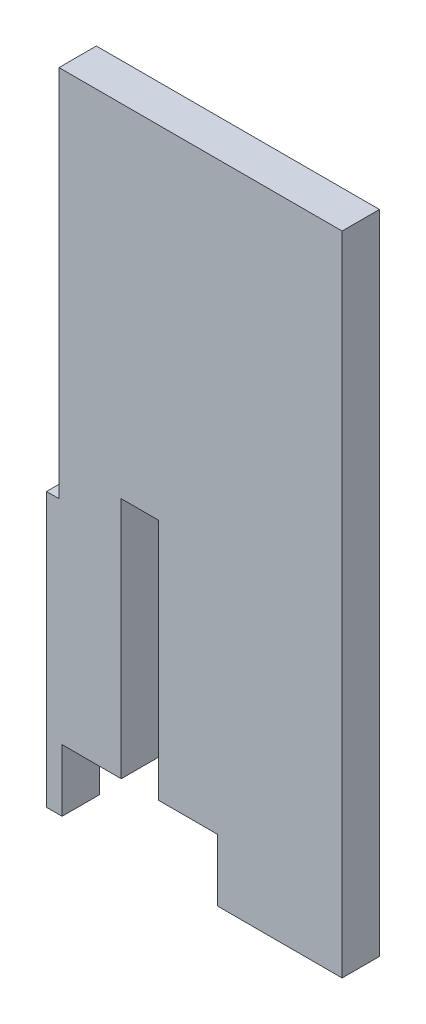
from build123d import *

# Parameters (mm, degrees)
BOSS_EXTRUDE1_DEPTH = 6
SKETCH3_W           = 6
SKETCH3_H           = 60
CUT_EXTRUDE1_DEPTH  = 10
CUT_EXTRUDE2_DEPTH  = 187.01085661


with BuildPart() as part:
    # Sketch1 → Boss-Extrude1 (new body)
    with BuildSketch(Plane.XY):
        Polygon((127.020625139, -33.445286794), (107.020625139, -33.445286794), (107.020625139, 70.514713206), (172.022422952, 70.514713206), (172.022422952, -33.445286794), (152.022422952, -33.445286794), (152.022422952, -23.465104548), (127.020625139, -23.465104548), align=None)
    extrude(amount=BOSS_EXTRUDE1_DEPTH)

    # Sketch3 → Cut-Extrude1 (cut)
    with BuildSketch(Plane(origin=(0, 0, 0), x_dir=(-1, 0, 0), z_dir=(0, 0, -1))):
        with Locations((-139.522422952, -14.485286794)):
            Rectangle(SKETCH3_W, SKETCH3_H)
    extrude(amount=-CUT_EXTRUDE1_DEPTH, mode=Mode.SUBTRACT)

    # Sketch4 → Cut-Extrude2 (cut, through all)
    with BuildSketch(Plane.XY.offset(6)):
        Polygon((124.522422952, -36.580409203), (107.020625139, -36.580409203), (107.020625139, 70.514713206), (120.512520278, 70.514713206), (126.522422952, 70.514713206), (126.522422952, 10.514713206), (124.522422952, 10.514713206), align=None)
    extrude(amount=-CUT_EXTRUDE2_DEPTH, mode=Mode.SUBTRACT)


solid = part.part
